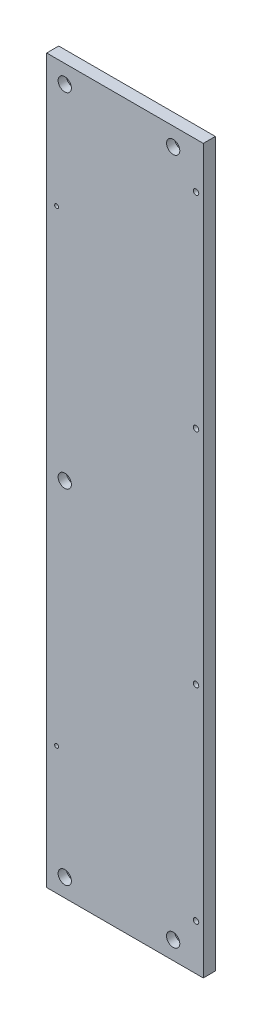
from build123d import *

# Parameters (mm, degrees)
SKETCH_1_W                  = 130
SKETCH_1_H                  = 600
EXTRUDE_1_DEPTH             = 10
HOLE_WIZARD_2_D             = 6.6
HOLE_WIZARD_2_CBORE_D       = 11
HOLE_WIZARD_2_CBORE_DEPTH   = 6.8
HOLE_WIZARD_M4_2_D          = 3.3
HOLE_WIZARD_2_2_D           = 4.5
HOLE_WIZARD_2_2_CBORE_D     = 8
HOLE_WIZARD_2_2_CBORE_DEPTH = 4.6


with BuildPart() as part:
    # 草图1 → 凸台-拉伸1 (new body)
    with BuildSketch(Plane.XY):
        Rectangle(SKETCH_1_W, SKETCH_1_H)
    extrude(amount=EXTRUDE_1_DEPTH)

    # Hole Wizard 2 (through all)
    with Locations(Plane.XY.offset(10)):
        with Locations((-50, 285), (-50, 0), (-50, -285), (40, 285), (40, -285)):
            CounterBoreHole(HOLE_WIZARD_2_D / 2, HOLE_WIZARD_2_CBORE_D / 2, HOLE_WIZARD_2_CBORE_DEPTH)

    # M4 螺纹孔2 (through all)
    with Locations(Plane.XY.offset(10)):
        with Locations((-56.75, 194), (-56.75, -194)):
            Hole(HOLE_WIZARD_M4_2_D / 2)

    # Hole Wizard 2 2 (through all)
    with Locations(Plane(origin=(0, 0, 0), x_dir=(-1, 0, 0), z_dir=(0, 0, -1))):
        with Locations((-59, -262), (-59, -92), (-59, 92), (-59, 262)):
            CounterBoreHole(HOLE_WIZARD_2_2_D / 2, HOLE_WIZARD_2_2_CBORE_D / 2, HOLE_WIZARD_2_2_CBORE_DEPTH)


solid = part.part
